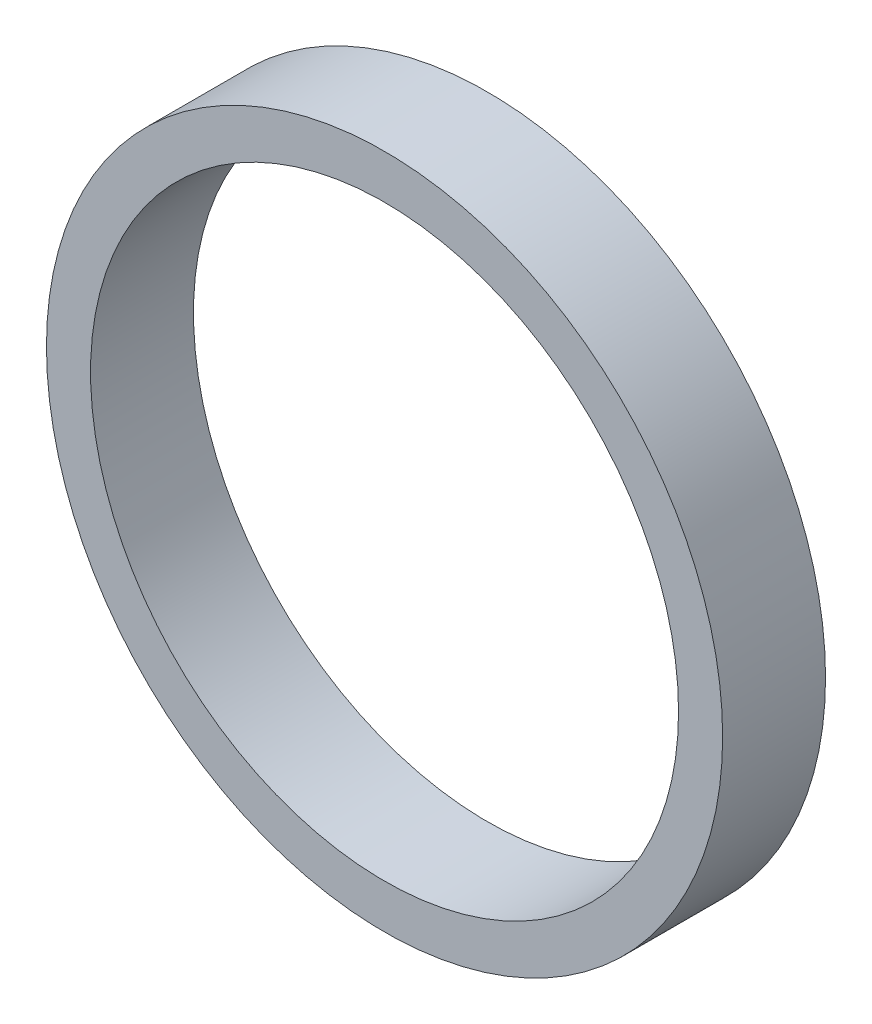
SolidWorks part; units mm, degrees
ref_plane "前视基准面" through (0, 0, 0) normal (0, 0, 1) x (1, 0, 0)
ref_plane "上视基准面" through (0, 0, 0) normal (0, 1, 0) x (1, 0, 0)
ref_plane "右视基准面" through (0, 0, 0) normal (1, 0, 0) x (0, 0, -1)
sketch "草图1" plane through (0, 0, 0) normal (0, 0, 1) x (1, 0, 0)
  circle A0 centre (0, 0) radius 20
  circle A1 centre (0, 0) radius 23
extrude "凸台-拉伸1" add sketch "草图1" along normal blind 7
